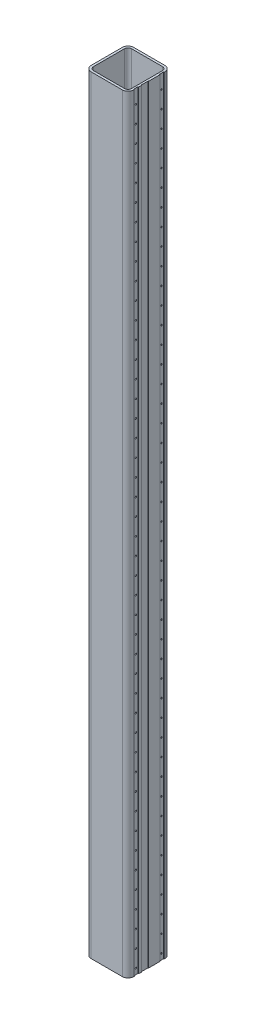
from build123d import *

# Parameters (mm, degrees)
BOSS_EXTRUDE1_DEPTH  = 1355
SKETCH2_W            = 2
SKETCH2_H            = 15
SKETCH2_W_2          = 1.5
SKETCH2_H_2          = 25
CUT_EXTRUDE1_DEPTH   = 4000
CUT_EXTRUDE2_REACH   = 1367.121
SKETCH4_R            = 2.6
LPATTERN2_COUNT      = 2
LPATTERN2_PITCH      = 90.4
LPATTERN2_COUNT_DIR2 = 45
LPATTERN2_PITCH_DIR2 = 60


with BuildPart() as part:
    # Sketch1 → Boss-Extrude1 (new, symmetric)
    with BuildSketch(Plane(origin=(0, 0, 0), x_dir=(1, 0, 0), z_dir=(0, 1, 0))):
        with BuildLine():
            Line((-55, -75), (55, -75))
            ThreePointArc((55, -75), (69.142135624, -69.142135624), (75, -55))
            Line((75, -55), (75, 55))
            ThreePointArc((75, 55), (69.142135624, 69.142135624), (55, 75))
            Line((55, 75), (-55, 75))
            ThreePointArc((-55, 75), (-69.142135624, 69.142135624), (-75, 55))
            Line((-75, 55), (-75, -55))
            ThreePointArc((-75, -55), (-69.142135624, -69.142135624), (-55, -75))
        make_face()
        with BuildLine():
            Line((-67, -55), (-67, 55))
            ThreePointArc((-67, 55), (-63.485281374, 63.485281374), (-55, 67))
            Line((-55, 67), (55, 67))
            ThreePointArc((55, 67), (63.485281374, 63.485281374), (67, 55))
            Line((67, 55), (67, -55))
            ThreePointArc((67, -55), (63.485281374, -63.485281374), (55, -67))
            Line((55, -67), (-55, -67))
            ThreePointArc((-55, -67), (-63.485281374, -63.485281374), (-67, -55))
        make_face(mode=Mode.SUBTRACT)
    extrude(amount=BOSS_EXTRUDE1_DEPTH, both=True)

    # Sketch2 → Cut-Extrude1 (cut)
    with BuildSketch(Plane.XZ.offset(1355)):
        with Locations((74, 45.2)):
            Rectangle(SKETCH2_W, SKETCH2_H)
        with Locations((74, -45.2)):
            Rectangle(SKETCH2_W, SKETCH2_H)
        with Locations((74.25, 14.7)):
            Rectangle(SKETCH2_W_2, SKETCH2_H_2)
    extrude(amount=-CUT_EXTRUDE1_DEPTH, mode=Mode.SUBTRACT)

    # Sketch4 → Cut-Extrude2 (cut, up to next)
    with BuildSketch(Plane(origin=(73, 0, 0), x_dir=(0, 0, -1), z_dir=(1, 0, 0)), mode=Mode.PRIVATE) as cut_extrude2_sk1:
        with Locations((-45.2, -1335)):
            Circle(SKETCH4_R)
    cut_extrude2_tool1 = extrude(cut_extrude2_sk1.sketch, amount=-CUT_EXTRUDE2_REACH, mode=Mode.PRIVATE) & part.part
    cut_extrude2 = cut_extrude2_tool1.solids().sort_by_distance((73, -1335, 45.2))[0]
    add(cut_extrude2, mode=Mode.SUBTRACT)

    # LPattern2: Cut-Extrude2 2 × 45
    with Locations(*[(0, j * LPATTERN2_PITCH_DIR2, -i * LPATTERN2_PITCH) for i in range(LPATTERN2_COUNT) for j in range(LPATTERN2_COUNT_DIR2) if (i, j) != (0, 0)]):
        add(cut_extrude2, mode=Mode.SUBTRACT)


solid = part.part
